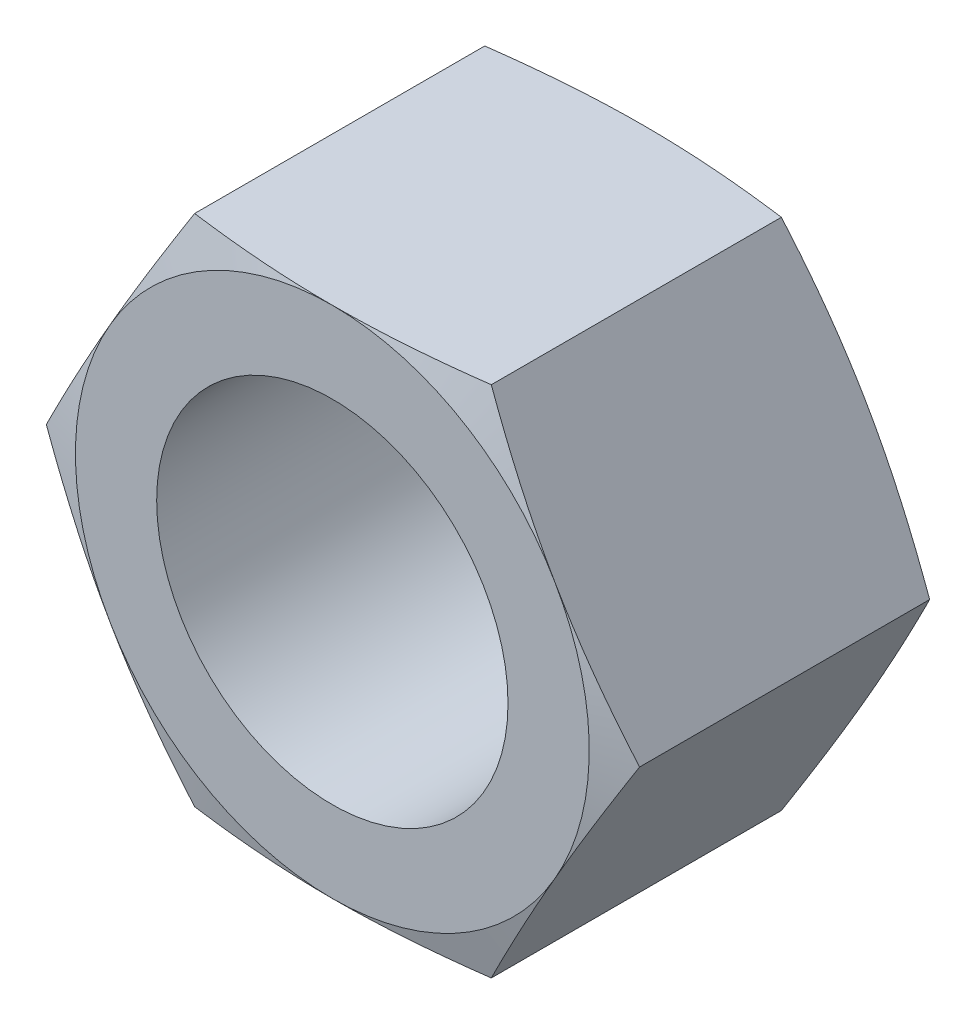
SolidWorks part; units mm, degrees
ref_plane "基准面1" through (0, 0, 0) normal (0, 0, 1) x (1, 0, 0)
ref_plane "基准面2" through (0, 0, 0) normal (0, 1, 0) x (1, 0, 0)
ref_plane "基准面3" through (0, 0, 0) normal (1, 0, 0) x (0, 0, -1)
sketch "尺寸草图" plane through (0, 0, 0) normal (0, 0, 1) x (1, 0, 0)
  line L0 (0, 0) -> (24.1005, 0)
  point P3 (36, 0)
  point P4 (1.5, 0)
  point P5 (60.79, 0)
  point P6 (31.9, 0)
  point P7 (6.4, 0)
  point P8 (55, 0)
sketch "草图1" plane through (0, 0, 0) normal (0, 0, 1) x (1, 0, 0)
  line L0 (-26.8088, 0) -> (37.1748, 0) construction
  line L1 (0, 25.0215) -> (0, -25.0215) construction
  line L3 (15.1975, 26.3228) -> (-15.1975, 26.3228)
  line L4 (-15.1975, 26.3228) -> (-30.395, 0)
  line L5 (-30.395, 0) -> (-15.1975, -26.3228)
  line L6 (-15.1975, -26.3228) -> (15.1975, -26.3228)
  line L7 (15.1975, -26.3228) -> (30.395, 0)
  line L8 (30.395, 0) -> (15.1975, 26.3228)
  circle A0 centre (0, 0) radius 26.3228 construction
  circle A1 centre (0, 0) radius 18
extrude "基体-拉伸" add sketch "草图1" along normal blind 31.9
cosmetic thread "装饰螺纹线1" parameters "D2"=37.8
sketch "草图2" plane through (0, 0, 0) normal (0, 0, -1) x (-1, 0, 0)
  line L0 (-15.1975, 26.3228) -> (15.1975, 26.3228) construction
  circle A0 centre (0, 0) radius 26.3228
  circle A1 centre (0, 0) radius 18 construction
extrude "切除-拉伸1" cut sketch "草图2" against normal blind 38 draft 75 flip side to cut
sketch "草图3" plane through (0, 0, 31.9) normal (0, 0, 1) x (1, 0, 0)
  line L0 (30.395, 0) -> (15.1975, 26.3228) construction
  circle A0 centre (0, 0) radius 26.3228
extrude "切除-拉伸2" cut sketch "草图3" against normal blind 38 draft 75 flip side to cut
chamfer "倒角1" [suppressed] distance 0.2 angle 45
equation "\"e@草图1\" = \"e@尺寸草图\""
equation "\"D@草图1\" = \"D@尺寸草图\""
equation "\"m@基体-拉伸\" = \"m@尺寸草图\""
equation "\"D2@装饰螺纹线1\" = 1.05 * \"D@尺寸草图\""
